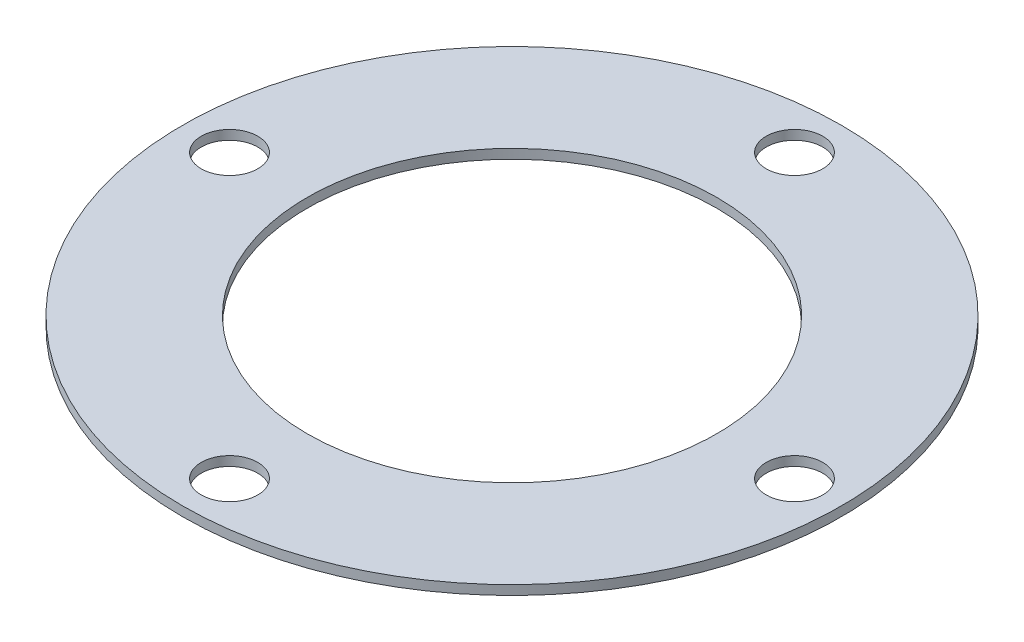
SolidWorks part; units mm, degrees
material "耐油橡胶Ⅰ- 2"
ref_plane "前视基准面" through (0, 0, 0) normal (0, 0, 1) x (1, 0, 0)
ref_plane "上视基准面" through (0, 0, 0) normal (0, 1, 0) x (1, 0, 0)
ref_plane "右视基准面" through (0, 0, 0) normal (1, 0, 0) x (0, 0, -1)
sketch "草图1" plane through (0, 0, 0) normal (0, 1, 0) x (1, 0, 0)
  circle A0 centre (0, 0) radius 70
  circle A1 centre (0, 0) radius 43.5
  dimension "D1" = 140
  dimension "D2" = 87
extrude "凸台-拉伸1" add sketch "草图1" along normal blind 2
sketch "草图3" plane through (0, 2, 0) normal (0, 1, 0) x (1, 0, 0)
  circle A0 centre (0, 0) radius 60 construction
  circle A1 centre (0, 60) radius 6
  circle A2 centre (60, 0) radius 6
  circle A3 centre (0, -60) radius 6
  circle A4 centre (-60, 0) radius 6
  point P14 (0, 0)
  dimension "D1" = 120
  dimension "D2" = 12
  dimension "D3" = 4
extrude "切除-拉伸1" cut sketch "草图3" against normal through all
